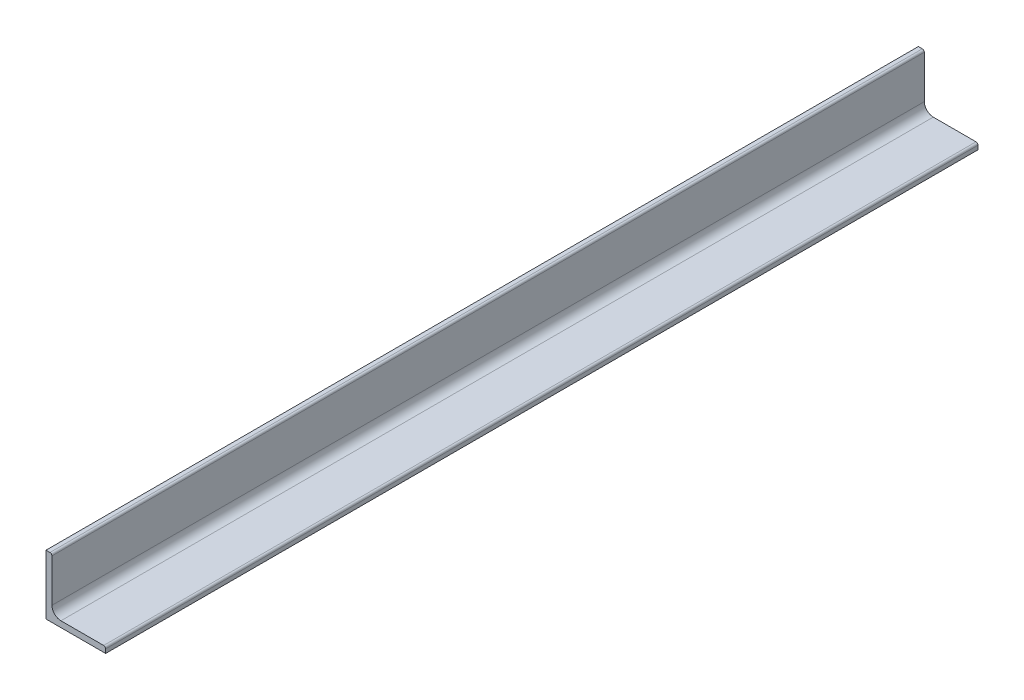
from build123d import *

# Parameters (mm, degrees)
BOSS_EXTRUDE1_DEPTH = 219.4


with BuildPart() as part:
    # Sketch1 → Boss-Extrude1 (new, symmetric)
    with BuildSketch(Plane.XY):
        with BuildLine():
            Line((0, 0), (0, 30))
            Line((0, 30), (2, 30))
            ThreePointArc((2, 30), (2.707106781, 29.707106781), (3, 29))
            Line((3, 29), (3, 7.5))
            ThreePointArc((3, 7.5), (4.318019485, 4.318019485), (7.5, 3))
            Line((7.5, 3), (29, 3))
            ThreePointArc((29, 3), (29.707106781, 2.707106781), (30, 2))
            Line((30, 2), (30, 0))
            Line((30, 0), (0, 0))
        make_face()
    extrude(amount=BOSS_EXTRUDE1_DEPTH, both=True)


solid = part.part
